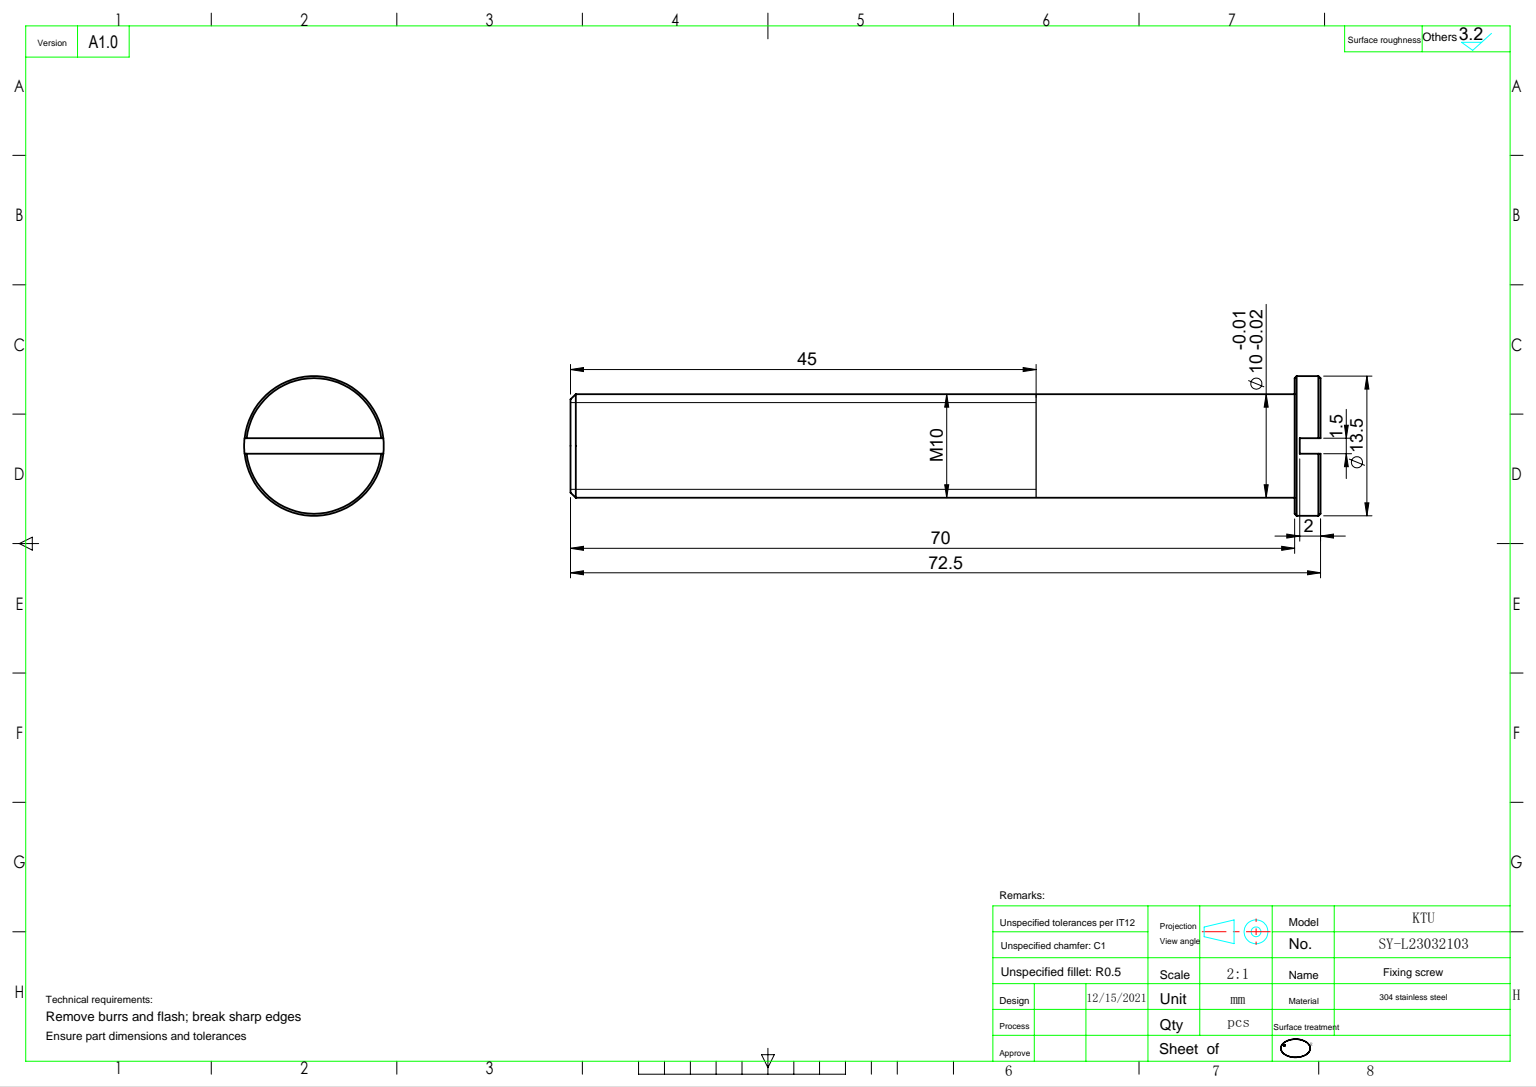
SolidWorks part; units mm, degrees
ref_plane "前视基准面" through (0, 0, 0) normal (0, 0, 1) x (1, 0, 0)
ref_plane "上视基准面" through (0, 0, 0) normal (0, 1, 0) x (1, 0, 0)
ref_plane "右视基准面" through (0, 0, 0) normal (1, 0, 0) x (0, 0, -1)
sketch "草图4" plane through (0, 0, 0) normal (0, 0, 1) x (1, 0, 0)
  circle A0 centre (0, 0) radius 5
  dimension "D1" = 10
extrude "凸台-拉伸3" add sketch "草图4" along normal blind 70
cosmetic thread "装饰螺纹线1" parameters "D1"=45, "D2"=8.376
sketch "草图5" plane through (0, 0, 0) normal (0, 0, -1) x (-1, 0, 0)
  circle A0 centre (0, 0) radius 6.75
  dimension "D1" = 13.5
extrude "凸台-拉伸4" add sketch "草图5" along normal blind 2.5
chamfer "倒角1" distance 0.5 angle 45 1 edges at (5, 0, 70)
chamfer "倒角2" distance 0.2 angle 45 2 edges at (-6.75, 0, 0) (-6.75, 0, -2.5)
sketch "草图6" plane through (0, 0, -2.5) normal (0, 0, -1) x (-1, 0, 0)
  line L1 (-7.5, 0.75) -> (7.5, 0.75)
  line L2 (-7.5, 0.75) -> (-7.5, -0.75)
  line L3 (-7.5, -0.75) -> (7.5, -0.75)
  line L4 (7.5, 0.75) -> (7.5, -0.75)
  line L5 (-7.5, 0.75) -> (7.5, -0.75) construction
  line L6 (-7.5, -0.75) -> (7.5, 0.75) construction
  point P0 (0, 0)
  dimension "D1" = 1.5
  dimension "D2" = 15
extrude "切除-拉伸1" cut sketch "草图6" against normal blind 2
